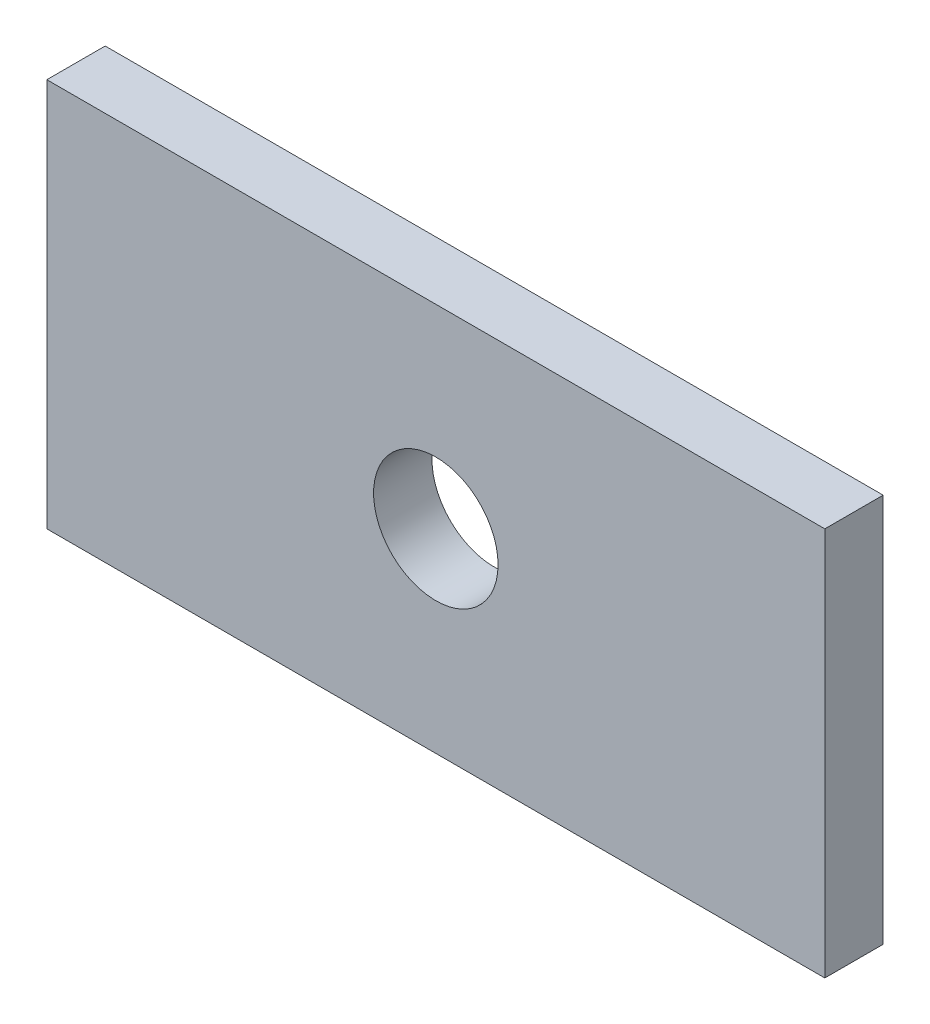
SolidWorks part; units mm, degrees
ref_plane "前视基准面" through (0, 0, 0) normal (0, 0, 1) x (1, 0, 0)
ref_plane "上视基准面" through (0, 0, 0) normal (0, 1, 0) x (1, 0, 0)
ref_plane "右视基准面" through (0, 0, 0) normal (1, 0, 0) x (0, 0, -1)
other "Configuration Table"
sketch "草图1" plane through (0, 0, 0) normal (0, 0, 1) x (1, 0, 0)
  line L0 (-20, -10) -> (20, -10)
  line L1 (20, -10) -> (20, 10)
  line L2 (20, 10) -> (-20, 10)
  line L3 (-20, 10) -> (-20, -10)
  point P0 (0, 0)
  dimension "D1" = 20
  dimension "D2" = 40
  dimension "D3" = 10
  dimension "D4" = 20
extrude "凸台-拉伸1" add sketch "草图1" against normal mid plane 3
sketch "草图2" plane through (0, 0, 0) normal (0, 0, 1) x (1, 0, 0)
  circle A0 centre (0, 0) radius 3.2
  point P0 (0, 0)
  dimension "D1" = 6.4
extrude "切除-拉伸1" cut sketch "草图2" against normal mid plane 23
